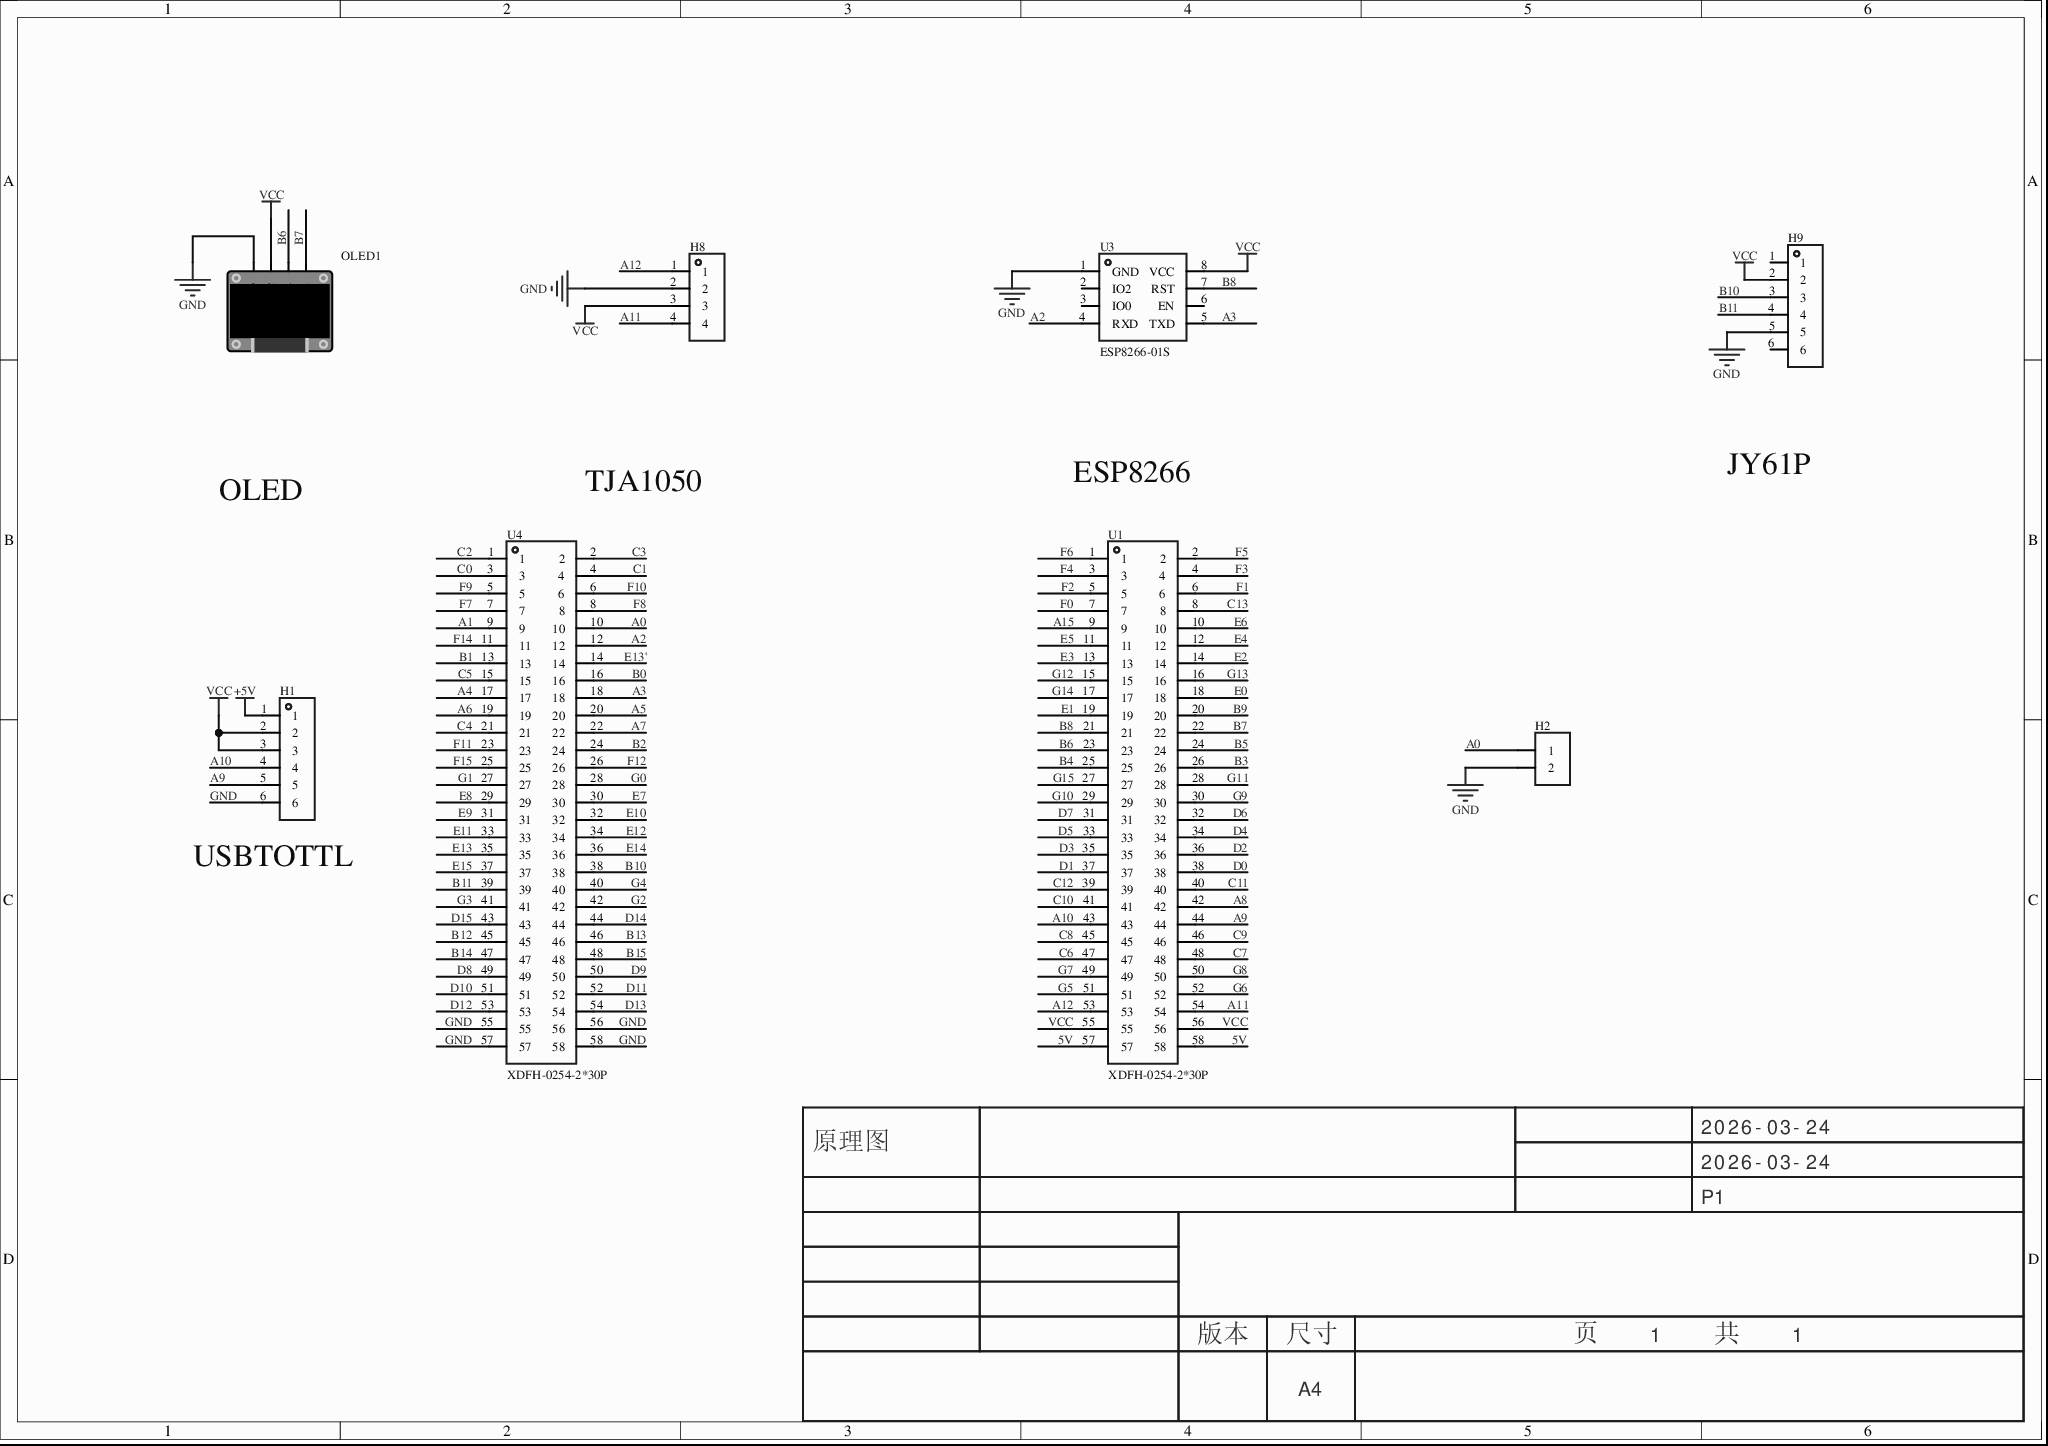
[diagram p0: MISC51816-3.schdoc]
# Altium project MISC51816-2.PrjPcb
1 sheet, 8 parts. Net scope: global (net labels, ports and power ports of the same name join across sheets).
Board file: MISC51816.pcbdoc

## Sheet MISC51816-3.schdoc
size 297 x 209 mm; Version: V1.0; @Project Name: MISC51816; @Page Count: 1; @Update Date: 2026-03-24; @Create Date: 2026-03-24; @Schematic Name: MISC51816; @Page No: 1; @Create Time: 18:58:15; @Update Time: 22:44:58; @Board Name: MISC51816

### Parts
H1  (no value)  [HDR-TH_6P-P2.54-V-F]
H2  (no value)  [HDR-TH_2P-P2.54-V-F]
H8  (no value)  [HDR-TH_4P-P2.54-V-F]
H9  (no value)  [HDR-TH_6P-P2.54-V-F]
OLED1  (no value)  [0.96OLED_4P]
U1  XDFH-0254-2*30P  [CONN-TH_60P-P2.54_LX_XDFH-0254-2X30P]
U3  ESP8266-01S  [WIFIM-TH_ESP8266-01S]
U4  XDFH-0254-2*30P  [CONN-TH_60P-P2.54_LX_XDFH-0254-2X30P]

### Nets
+5V: H1.1
GND: H1.6 H2.2 H8.2 H9.5 OLED1.1(GND) U3.1(GND) U4.55 U4.56 U4.57 U4.58
VCC: H1.2 H1.3 H8.3 H9.2 OLED1.2(VCC) U1.55 U1.56 U3.8(VCC)
5V: U1.57 U1.58
A0: H2.1 U4.10
A1: U4.9
A2: U3.4(RXD) U4.12
A3: U3.5(TXD) U4.18
A4: U4.17
A5: U4.20
A6: U4.19
A7: U4.22
A8: U1.42
A9: H1.5 U1.44
A10: H1.4 U1.43
A11: H8.4 U1.54
A12: H8.1 U1.53
A15: U1.9
B0: U4.16
B1: U4.13
B2: U4.24
B3: U1.26
B4: U1.25
B5: U1.24
B6: OLED1.3(SCL) U1.23
B7: OLED1.4(SDA) U1.22
B8: U1.21 U3.7(RST)
B9: U1.20
B10: H9.3 U4.38
B11: H9.4 U4.39
B12: U4.45
B13: U4.46
B14: U4.47
B15: U4.48
C0: U4.3
C1: U4.4
C2: U4.1
C3: U4.2
C4: U4.21
C5: U4.15
C6: U1.47
C7: U1.48
C8: U1.45
C9: U1.46
C10: U1.41
C11: U1.40
C12: U1.39
C13: U1.8
D0: U1.38
D1: U1.37
D2: U1.36
D3: U1.35
D4: U1.34
D5: U1.33
D6: U1.32
D7: U1.31
D8: U4.49
D9: U4.50
D10: U4.51
D11: U4.52
D12: U4.53
D13: U4.54
D14: U4.44
D15: U4.43
E0: U1.18
E1: U1.19
E2: U1.14
E3: U1.13
E4: U1.12
E5: U1.11
E6: U1.10
E7: U4.30
E8: U4.29
E9: U4.31
E10: U4.32
E11: U4.33
E12: U4.34
E13: U4.35
E13': U4.14
E14: U4.36
E15: U4.37
F0: U1.7
F1: U1.6
F2: U1.5
F3: U1.4
F4: U1.3
F5: U1.2
F6: U1.1
F7: U4.7
F8: U4.8
F9: U4.5
F10: U4.6
F11: U4.23
F12: U4.26
F14: U4.11
F15: U4.25
G0: U4.28
G1: U4.27
G2: U4.42
G3: U4.41
G4: U4.40
G5: U1.51
G6: U1.52
G7: U1.49
G8: U1.50
G9: U1.30
G10: U1.29
G11: U1.28
G12: U1.15
G13: U1.16
G14: U1.17
G15: U1.27

Not connected (* = marked no-connect by the designer): H9 1 6; U3 2(IO2) 3(IO0) 6(EN)

### Notes on the sheet
- OLED
- (near U4) TJA1050
- ESP8266
- JY61P
- (near H1) USBTOTTL
- 2026-03-24
- 原理图
- P1
- 版本
- 尺寸
- A4
- 页    1    共    1

### Library data of the parts
H1 H9 = HDR-F_2.54_1x6P: Symbol: Header-Female-2.54_1x6; 3D Model: 0f5bcf94dcda47d085f24cdca1696fe9; 3D Model Transform: 619.684,94.488,0,0,0,0,0,0,-125.984; ConvertToPcb: yes; Device: HDR-F_2.54_1x6P; Supplier Part: C40877; Supplier Footprint: 插件; AddInBom: yes; FootprintName: HDR-TH_6P-P2.54-V-F; ModelName: HDR-TH_6P-P2.54-V-F
H2 = HDR-F_2.54_1x2P: Symbol: Header-Female-2.54_1x2; ConvertToPcb: yes; ModelId: a9450ef445564560a104363b9aacde4e0819f05c4eef4c71ace90d822a990e87; ModelName: HDR-TH_2P-P2.54-F-LI-1X2P; ModelTransform: 215.7476,98.425,0,0,0,0,0,0,-129.921; Device: HDR-F_2.54_1x2P; AddInBom: yes; SupplierPart: C49661; Supplier Footprint: 插件; FootprintName: HDR-TH_2P-P2.54-V-F
H8 = HDR-F_2.54_1x4P: Symbol: 2.54-1*4P母; 3D Model: d187812051054f85879fcaa51a310d8e; 3D Model Transform: 419.6842,98.464,0,0,0,0,0,0,-118.11; ConvertToPcb: yes; Device: HDR-F_2.54_1x4P; Supplier Part: C2718488; Supplier Footprint: 插件; AddInBom: yes; FootprintName: HDR-TH_4P-P2.54-V-F; ModelName: HDR-TH_4P-P2.54-V-F
OLED1 = 0.96OLED模块_4P: ConvertToPcb: yes; ModelId: 79c000fdb68d45a296c2e9bedf4f9055; ModelTransform: 1393.69792,1318.895,0,0,0,0,0,-560.079,-137.795; Symbol: 0.96OLED模块_4P; Device: 0.96OLED模块_4P; AddInBom: yes; FootprintName: 0.96OLED_4P; Supplier Footprint: 插件; ModelName: 0.96OLED_4P
U1 U4 = XDFH-0254-2*30P: 连接器类型:简牛座;间距:2.54mm;结构:2x30P;额定电流:3A;额定电压:500V;封装形式:直插;排数:2;每排PIN数:30;触头材质:铜;触头镀层:金;工作温度范围:-45℃~+105℃;焊接温度(最大值):260℃;; Manufacturer: LX(连欣科技); AddInBom: yes; ModelId: a26cd603bfef41ef9c4646cffd18b6cf0819f05c4eef4c71ace90d822a990e87; ModelTransform: 3299.20616,350.7867,0,180,0,0,0,3.937,-125.984; Connector Type: 简牛座; Pitch: 2.54mm; Structure: 2x30P; Current Rating (Max): 3A; Voltage Rating (Max): 500V; Holder Type: 直插; Pin Number in each Row: 30; Soldering Temperature(Max): 260℃; Symbol: XDFH-0254-2*30P; Device: XDFH-0254-2*30P; LCSC Part Name: 镀2U全金品质简牛插座PH2.54MM-2*30PIN直插板 DIP; SupplierPart: C19193817; ManufacturerPart: XDFH-0254-2*30P; Supplier Footprint: 插件,P=2.54mm; JLCPCB Part Class: Extended Part; Datasheet: https://atta.szlcsc.com/upload/public/pdf/source/20231117/B05B179C28F8598ADEE3EE3DBCADEC41.pdf; Supplier: LCSC; ConvertToPcb: yes; FootprintName: CONN-TH_60P-P2.54_LX_XDFH-0254-2X30P; ModelName: CONN-TH_60P-P2.54_LX_XDFH-0254-2X30P; Number of Rows: 2; Contact Material: 铜; Contact Plating: 金; Operating Temperature Range: -45℃~+105℃
U3 = ESP8266-01S: AddInBom: yes; ModelId: 7671a3a19d0d4245ae5d5806b59f4d510819f05c4eef4c71ace90d822a990e87; ModelTransform: 566.928,972.439,0,0,0,0,0,378.464,-118.11; Symbol: ESP8266-01S; Device: ESP8266-01S; LCSC Part Name: ESP8266-01S; SupplierPart: C9900150497; ManufacturerPart: ESP8266-01S; Supplier Footprint: TH-8P; JLCPCB Part Class: Extended Part; Supplier: LCSC; ConvertToPcb: yes; FootprintName: WIFIM-TH_ESP8266-01S; ModelName: WIFIM-TH_ESP8266-01S